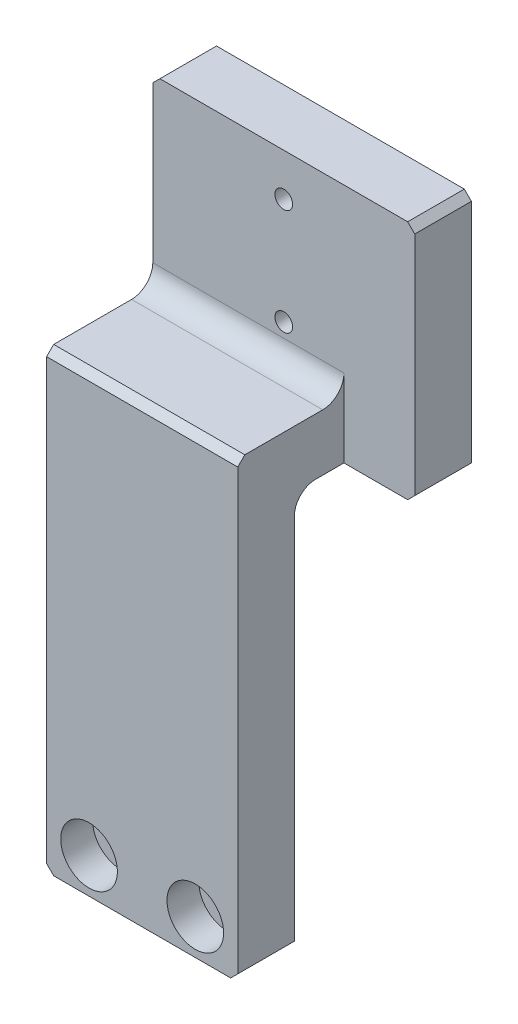
from build123d import *

# Parameters (mm, degrees)
SKETCH1_W                               = 37
SKETCH1_H                               = 90
BOSS_EXTRUDE1_DEPTH                     = 4
SKETCH6_W                               = 37
SKETCH6_H                               = 34
BOSS_EXTRUDE2_DEPTH                     = 15
M3_TAPPED_HOLE1_D                       = 2.5
CBORE_FOR_M4_HEX_HEAD_BOLT1_D           = 4.5
CBORE_FOR_M4_HEX_HEAD_BOLT1_CBORE_D     = 8
CBORE_FOR_M4_HEX_HEAD_BOLT1_CBORE_DEPTH = 4.5
SKETCH7_W                               = 15
SKETCH7_H                               = 26
CUT_EXTRUDE1_DEPTH                      = 100.146356464
CUT_EXTRUDE2_REACH                      = 101.99
SKETCH8_W                               = 10
SKETCH8_H                               = 64
FILLET1_R                               = 3
CHAMFER1_SIZE                           = 1
CHAMFER2_SIZE                           = 1


with BuildPart() as part:
    # Sketch1 → Boss-Extrude1 (new, symmetric)
    with BuildSketch(Plane.XY):
        with Locations((18.5, -45)):
            Rectangle(SKETCH1_W, SKETCH1_H)
    extrude(amount=BOSS_EXTRUDE1_DEPTH, both=True)

    # Sketch6 → Boss-Extrude2 (add)
    with BuildSketch(Plane.XY.offset(-4)):
        with Locations((18.5, -17)):
            Rectangle(SKETCH6_W, SKETCH6_H)
    extrude(amount=-BOSS_EXTRUDE2_DEPTH)

    # M3 Tapped Hole1 (through all)
    with Locations(Plane.XY.offset(4)):
        with Locations((18.5, -21), (18.5, -6)):
            Hole(M3_TAPPED_HOLE1_D / 2)

    # CBORE for M4 Hex Head Bolt1 (through all)
    with Locations(Plane.XY.offset(4)):
        with Locations((6, -85), (21, -85)):
            CounterBoreHole(CBORE_FOR_M4_HEX_HEAD_BOLT1_D / 2, CBORE_FOR_M4_HEX_HEAD_BOLT1_CBORE_D / 2, CBORE_FOR_M4_HEX_HEAD_BOLT1_CBORE_DEPTH)

    # Sketch7 → Cut-Extrude1 (cut, through all)
    with BuildSketch(Plane(origin=(37, 0, 0), x_dir=(0, 0, -1), z_dir=(1, 0, 0))):
        with Locations((3.5, -13)):
            Rectangle(SKETCH7_W, SKETCH7_H)
    extrude(amount=-CUT_EXTRUDE1_DEPTH, mode=Mode.SUBTRACT)

    # Cut-Extrude2: up to this face of the body (flat: up to its plane)
    cut_extrude2_end = Plane(part.part.faces().sort_by_distance((18.5, -12.99484475, -11))[0])
    # Sketch8 → Cut-Extrude2 (cut, up to the picked face)
    with BuildSketch(Plane.XY.offset(4), mode=Mode.PRIVATE) as cut_extrude2_sk1:
        with Locations((32, -58)):
            Rectangle(SKETCH8_W, SKETCH8_H)
    cut_extrude2_tool1 = split(extrude(cut_extrude2_sk1.sketch, amount=-CUT_EXTRUDE2_REACH, mode=Mode.PRIVATE), bisect_by=cut_extrude2_end, keep=Keep.BOTH, mode=Mode.PRIVATE)
    add(cut_extrude2_tool1.solids().sort_by(Axis((32, -58, 4), (0, 0, -1)))[0], mode=Mode.SUBTRACT)

    # Fillet1
    fillet1_edges = [part.edges().sort_by_distance(p)[0] for p in [
        (13.5, -34, -4),
        (13.5, -26, -11),
    ]]
    fillet(fillet1_edges, radius=FILLET1_R)

    # Chamfer1
    chamfer1_edges = [part.edges().sort_by_distance(p)[0] for p in [
        (37, -34, -15),
        (37, 0, -15),
        (0, 0, -15),
        (0, -90, 0),
        (27, -90, 0),
    ]]
    chamfer(chamfer1_edges, length=CHAMFER1_SIZE)

    # Chamfer2
    chamfer2_edges = [part.edges().sort_by_distance(p)[0] for p in [
        (13.5, -26, 4),
        (18, -34, -19),
    ]]
    chamfer(chamfer2_edges, length=CHAMFER2_SIZE)


solid = part.part
